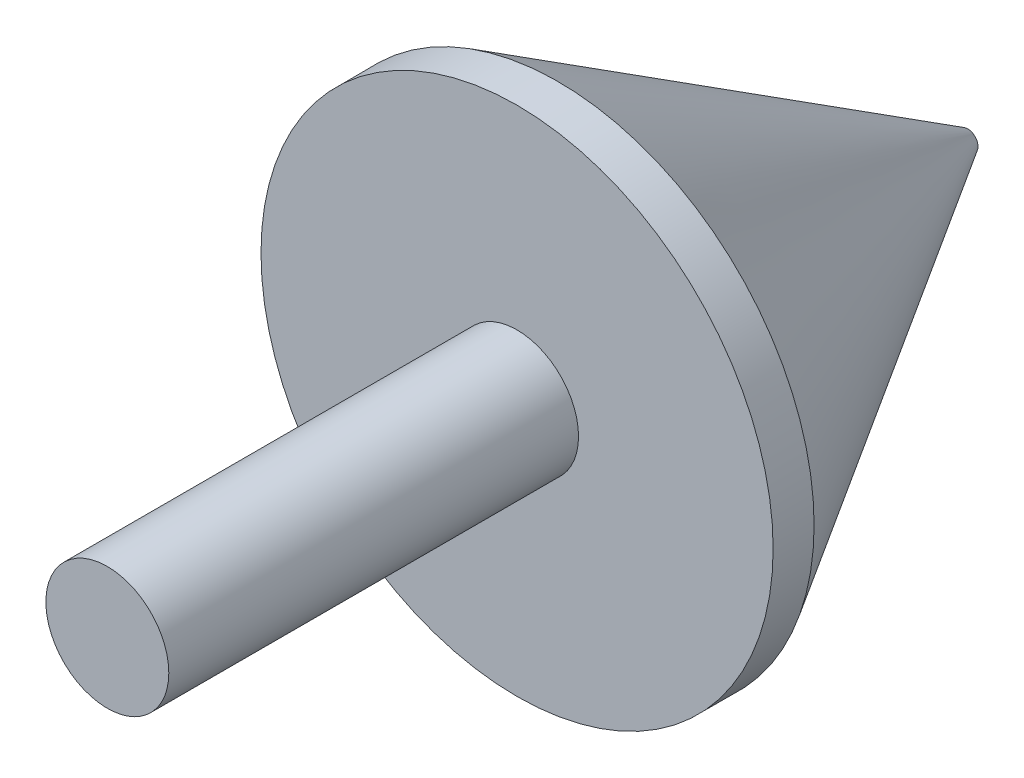
SolidWorks part; units mm, degrees
ref_plane "Front Plane" through (0, 0, 0) normal (0, 0, 1) x (1, 0, 0)
ref_plane "Top Plane" through (0, 0, 0) normal (0, 1, 0) x (1, 0, 0)
ref_plane "Right Plane" through (0, 0, 0) normal (1, 0, 0) x (0, 0, -1)
sketch "Sketch1" plane through (0, 0, 0) normal (0, 0, 1) x (1, 0, 0)
  circle A0 centre (0, 0) radius 3
  dimension "D1" = 6
extrude "Boss-Extrude1" add sketch "Sketch1" along normal blind 20
sketch "Sketch2" plane through (0, 0, 0) normal (0, 0, -1) x (-1, 0, 0)
  circle A0 centre (0, 0) radius 12.5
  dimension "D1" = 25
extrude "Boss-Extrude2" add sketch "Sketch2" along normal blind 2
sketch "Sketch3" plane through (0, 0, 0) normal (0, 1, 0) x (1, 0, 0)
  line L0 (-12.5, 2) -> (-0.5, 22)
  line L2 (12.5, 2) -> (-12.5, 2) construction
  line L3 (0, 2) -> (-12.5, 2)
  line L4 (-0.5, 22) -> (0, 22)
  line L5 (0, 22) -> (0, 2)
  dimension "D1" = 20
  dimension "D2" = 12
  dimension "D3" = 0.5
revolve "Revolve2" add sketch "Sketch3" angle 360 about L5
